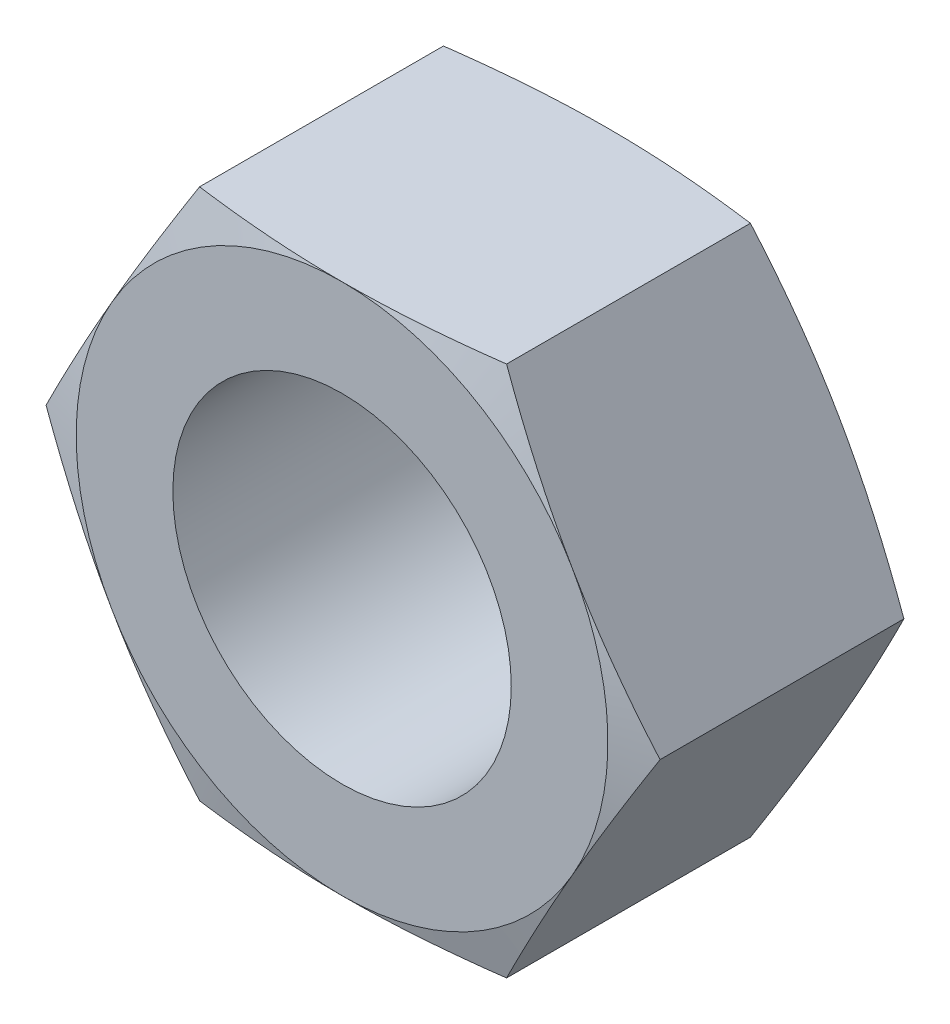
SolidWorks part; units mm, degrees
material "4级"
ref_plane "Plane1" through (0, 0, 0) normal (0, 0, 1) x (1, 0, 0)
ref_plane "Plane2" through (0, 0, 0) normal (0, 1, 0) x (1, 0, 0)
ref_plane "Plane3" through (0, 0, 0) normal (1, 0, 0) x (0, 0, -1)
sketch "Dimension sketch" plane through (0, 0, 0) normal (0, 0, 1) x (1, 0, 0)
  line L0 (0, 0) -> (24.1005, 0)
  point P3 (14, 0)
  point P4 (1.5, 0)
  point P5 (22.78, 0)
  point P6 (13.9, 0)
  point P7 (6.4, 0)
  point P8 (21, 0)
sketch "Sketch1" plane through (0, 0, 0) normal (0, 0, 1) x (1, 0, 0)
  line L0 (-26.8088, 0) -> (37.1748, 0) construction
  line L1 (0, 25.0215) -> (0, -25.0215) construction
  line L3 (6.35, 10.9985) -> (-6.35, 10.9985)
  line L4 (-6.35, 10.9985) -> (-12.7, 0)
  line L5 (-12.7, 0) -> (-6.35, -10.9985)
  line L6 (-6.35, -10.9985) -> (6.35, -10.9985)
  line L7 (6.35, -10.9985) -> (12.7, 0)
  line L8 (12.7, 0) -> (6.35, 10.9985)
  circle A0 centre (0, 0) radius 10.9985 construction
  circle A1 centre (0, 0) radius 7
extrude "Base-Extrude" add sketch "Sketch1" along normal blind 11
cosmetic thread "Cosmetic Thread1" parameters "D2"=14.7
sketch "Sketch2" plane through (0, 0, 0) normal (0, 0, -1) x (-1, 0, 0)
  line L0 (-6.35, 10.9985) -> (6.35, 10.9985) construction
  circle A0 centre (0, 0) radius 10.9985
  circle A1 centre (0, 0) radius 7 construction
extrude "Cut-Extrude1" cut sketch "Sketch2" against normal blind 38 draft 75 flip side to cut
sketch "Sketch3" plane through (0, 0, 11) normal (0, 0, 1) x (1, 0, 0)
  line L0 (12.7, 0) -> (6.35, 10.9985) construction
  circle A0 centre (0, 0) radius 10.9985
extrude "Cut-Extrude2" cut sketch "Sketch3" against normal blind 38 draft 75 flip side to cut
chamfer "Chamfer1" [suppressed] distance 0.2 angle 45
equation "\"D@Sketch1\" = \"D@Dimension sketch\""
equation "\"D2@Cosmetic Thread1\" = 1.05 * \"D@Dimension sketch\""
